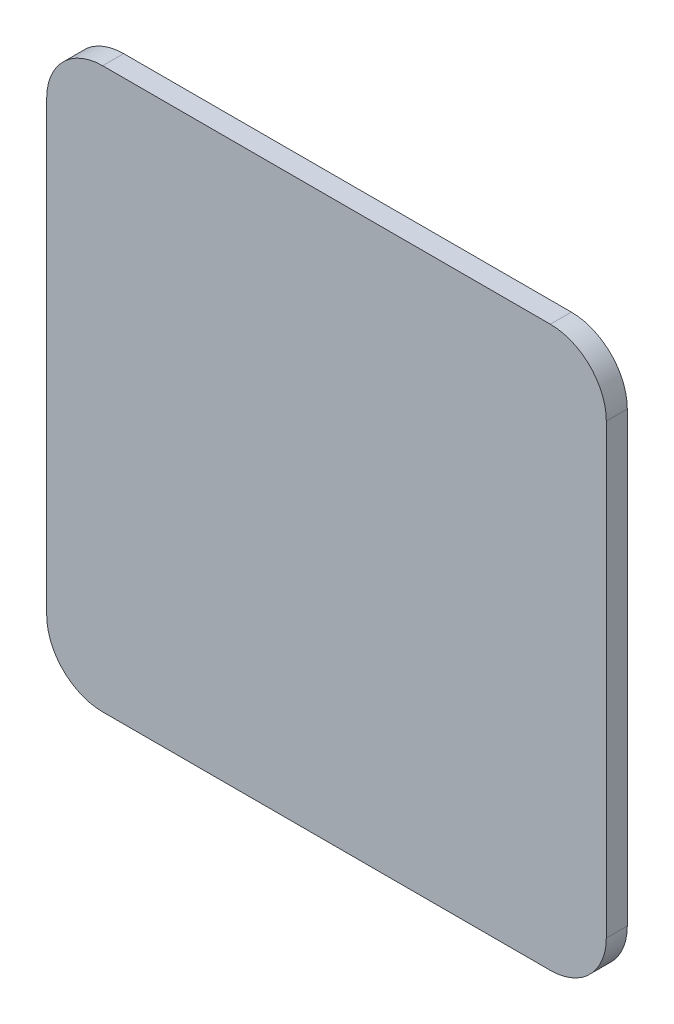
SolidWorks part; units mm, degrees
material "Q235A"
ref_plane "Front Plane" through (0, 0, 0) normal (0, 0, 1) x (1, 0, 0)
ref_plane "Top Plane" through (0, 0, 0) normal (0, 1, 0) x (1, 0, 0)
ref_plane "Right Plane" through (0, 0, 0) normal (1, 0, 0) x (0, 0, -1)
sketch "Sketch1" plane through (0, 0, 0) normal (0, 0, 1) x (1, 0, 0)
  line L1 (4, 0) -> (36, 0)
  line L2 (0, 4) -> (0, 36)
  line L3 (4, 40) -> (36, 40)
  line L4 (40, 4) -> (40, 36)
  arc A0 (0, 4) -> (4, 0) centre (4, 4) ccw
  arc A1 (36, 0) -> (40, 4) centre (36, 4) ccw
  arc A2 (40, 36) -> (36, 40) centre (36, 36) ccw
  arc A3 (4, 40) -> (0, 36) centre (4, 36) ccw
  point P7 (0, 0)
  point P12 (40, 40)
  point P15 (0, 40)
  dimension "D3" = 4
  dimension "D1" = 40
  dimension "D2" = 40
extrude "Boss-Extrude1" add sketch "Sketch1" along normal blind 1.5
